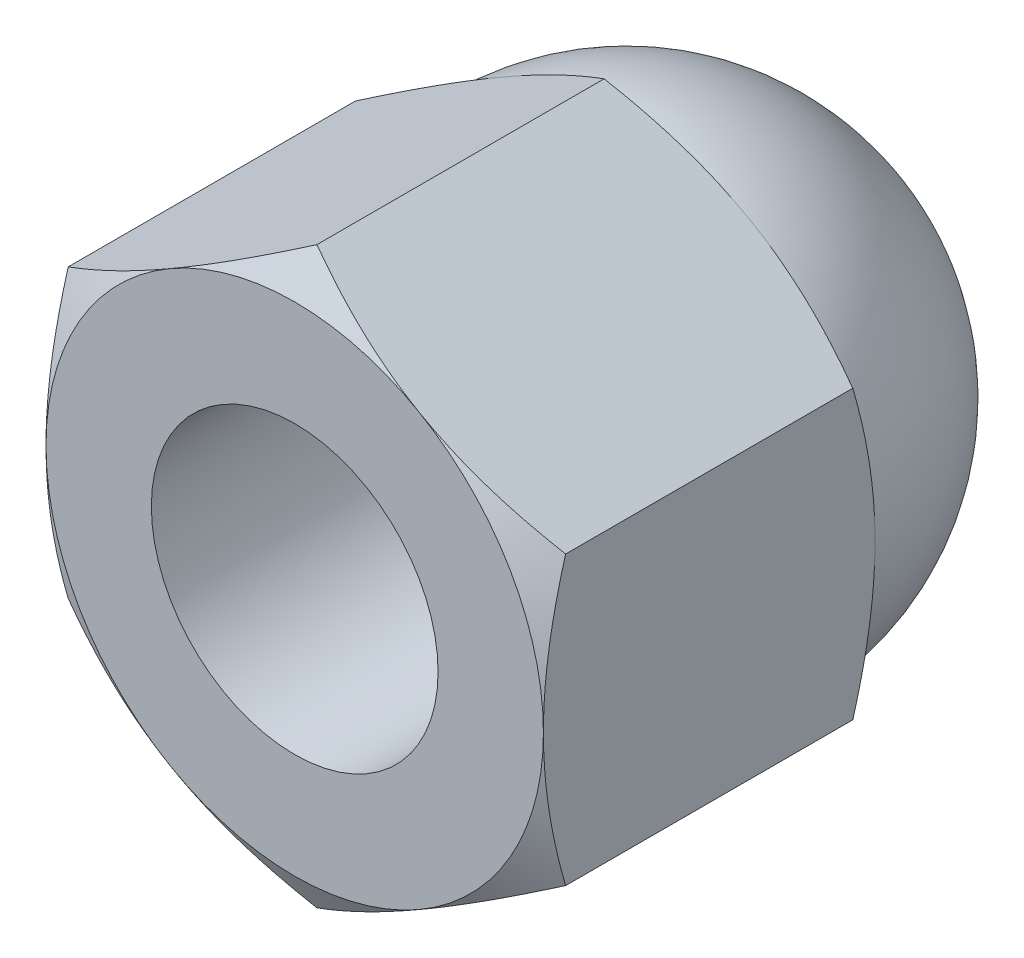
from build123d import *

# Parameters (mm, degrees)
EXTRUDE_575_DEPTH   = 12
SKETCH_4_OUTSIDE_W  = 93.598
SKETCH_4_OUTSIDE_H  = 96.382
SKETCH_4_OUTSIDE_R  = 9
CUT_EXTRUDE_1_DEPTH = 19.248287591
CUT_EXTRUDE_1_DRAFT = -60
SKETCH_5_OUTSIDE_W  = 117.332
SKETCH_5_OUTSIDE_H  = 120.116
SKETCH_5_OUTSIDE_R  = 9
CUT_EXTRUDE_2_DEPTH = 26.099800796
CUT_EXTRUDE_2_DRAFT = -60
SKETCH_6_R          = 5.188125
CUT_EXTRUDE_3_DEPTH = 10


with BuildPart() as part:
    # 草图1 → Extrude 575 (new body)
    with BuildSketch(Plane.XY):
        Polygon((0, 10.392304845), (-9, 5.196152423), (-9, -5.196152423), (0, -10.392304845), (9, -5.196152423), (9, 5.196152423), align=None)
    extrude(amount=EXTRUDE_575_DEPTH)

    # 草图2 → 凸台-旋转1 (revolve)
    with BuildSketch(Plane(origin=(0, 0, 0), x_dir=(1, 0, 0), z_dir=(0, 1, 0))):
        with BuildLine():
            Line((0, 9), (0, 0))
            Line((0, 0), (9, 0))
            ThreePointArc((9, 0), (6.363961031, 6.363961031), (0, 9))
        make_face()
    revolve(axis=Axis((0, 0, -2.579649935), (0, 0, 1)))


with BuildPart() as cut_extrude_1_tool:
    # 草图4 outside → 切除-拉伸1 (with draft: the straight prism first)
    with BuildSketch(Plane(origin=(0, 0, 0), x_dir=(-1, 0, 0), z_dir=(0, 0, -1))):
        Rectangle(SKETCH_4_OUTSIDE_W, SKETCH_4_OUTSIDE_H)
        Circle(SKETCH_4_OUTSIDE_R, mode=Mode.SUBTRACT)
    extrude(amount=-CUT_EXTRUDE_1_DEPTH)
    # 切除-拉伸1: the draft: its side faces are tilted about the plane it starts from
    cut_extrude_1_sides = [cut_extrude_1_tool.faces().sort_by_distance(p)[0] for p in [
        (0, -48.191, 9.624143795),
        (-46.799, 0, 9.624143795),
        (0, 48.191, 9.624143795),
        (46.799, 0, 9.624143795),
        (9, 0, 9.624143795),
    ]]
    draft(cut_extrude_1_sides, Plane(origin=(0, 0, 0), x_dir=(-1, 0, 0), z_dir=(0, 0, -1)), CUT_EXTRUDE_1_DRAFT)


with BuildPart() as part_1:
    add(part.part)

    # 切除-拉伸1: cut by cut_extrude_1_tool
    add(cut_extrude_1_tool.part, mode=Mode.SUBTRACT)


with BuildPart() as cut_extrude_2_tool:
    # 草图5 outside → 切除-拉伸2 (with draft: the straight prism first)
    with BuildSketch(Plane.XY.offset(12)):
        Rectangle(SKETCH_5_OUTSIDE_W, SKETCH_5_OUTSIDE_H)
        Circle(SKETCH_5_OUTSIDE_R, mode=Mode.SUBTRACT)
    extrude(amount=-CUT_EXTRUDE_2_DEPTH)
    # 切除-拉伸2: the draft: its side faces are tilted about the plane it starts from
    cut_extrude_2_sides = [cut_extrude_2_tool.faces().sort_by_distance(p)[0] for p in [
        (0, -60.058, -1.049900398),
        (58.666, 0, -1.049900398),
        (0, 60.058, -1.049900398),
        (-58.666, 0, -1.049900398),
        (-9, 0, -1.049900398),
    ]]
    draft(cut_extrude_2_sides, Plane.XY.offset(12), CUT_EXTRUDE_2_DRAFT)


with BuildPart() as part_2:
    add(part_1.part)

    # 切除-拉伸2: cut by cut_extrude_2_tool
    add(cut_extrude_2_tool.part, mode=Mode.SUBTRACT)

    # 草图6 → 切除-拉伸3 (cut)
    with BuildSketch(Plane.XY.offset(12)):
        Circle(SKETCH_6_R)
    extrude(amount=-CUT_EXTRUDE_3_DEPTH, mode=Mode.SUBTRACT)


solid = part_2.part
